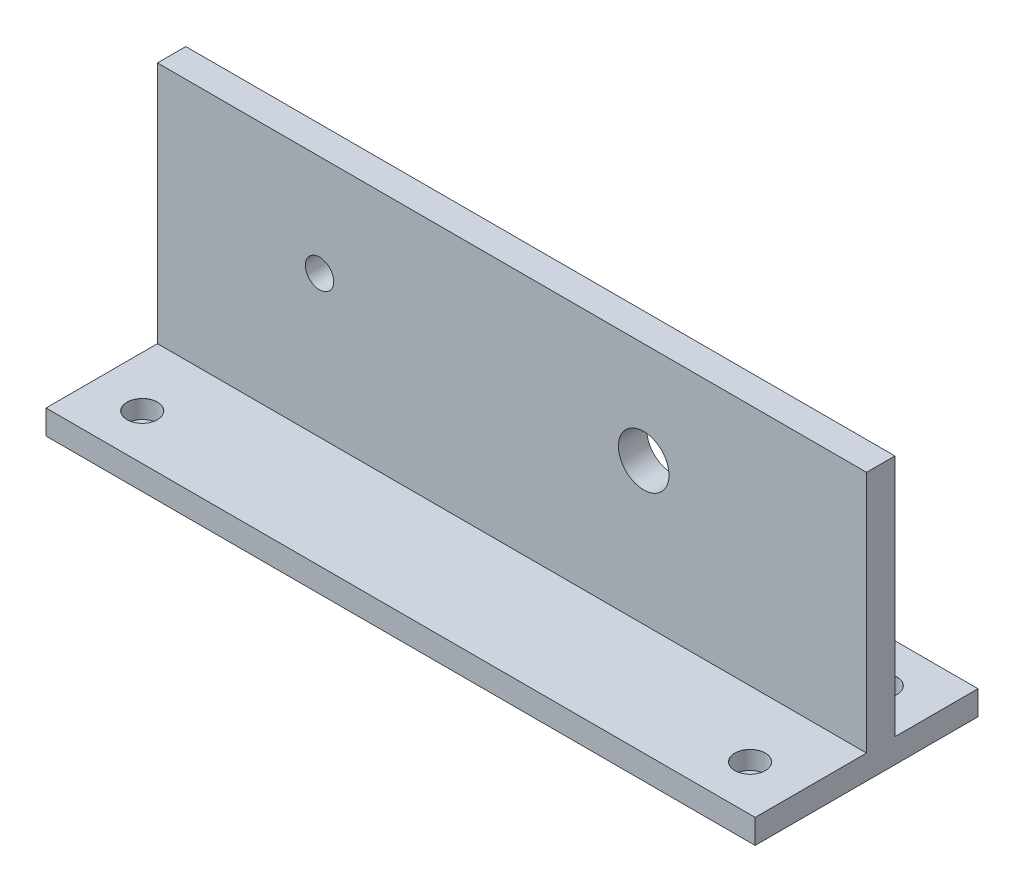
from build123d import *

# Parameters (mm, degrees)
SKETCH1_W                                    = 350
SKETCH1_H                                    = 110
BOSS_EXTRUDE1_DEPTH                          = 12
SKETCH2_W                                    = 350
SKETCH2_H                                    = 14
BOSS_EXTRUDE2_DEPTH                          = 120
CBORE_FOR_M8_HEXAGON_SOCKET_HEAD_CAP_2_COUNT = 2
CBORE_FOR_M8_HEXAGON_SOCKET_HEAD_CAP_2_PITCH = 65
CBORE_FOR_M8_HEXAGON_SOCKET_HEAD_CAP_3_COUNT = 2
CBORE_FOR_M8_HEXAGON_SOCKET_HEAD_CAP_3_PITCH = 300
CBORE_FOR_M8_HEXAGON_SOCKET_HEAD_CAP_4_COUNT = 2
CBORE_FOR_M8_HEXAGON_SOCKET_HEAD_CAP_4_PITCH = 306.960909563
CUT_EXTRUDE1_DEPTH                           = 230.804264538
CUT_EXTRUDE1_DEPTH_BACK                      = 230.804264538
SKETCH6_R                                    = 7
CUT_EXTRUDE2_DEPTH                           = 230.804264538
CUT_EXTRUDE2_DEPTH_BACK                      = 230.804264538
SKETCH7_R                                    = 12.5


with BuildPart() as part:
    # Sketch1 → Boss-Extrude1 (new body)
    with BuildSketch(Plane(origin=(0, 0, 0), x_dir=(1, 0, 0), z_dir=(0, 1, 0))):
        Rectangle(SKETCH1_W, SKETCH1_H)
    extrude(amount=BOSS_EXTRUDE1_DEPTH)

    # Sketch2 → Boss-Extrude2 (add)
    with BuildSketch(Plane(origin=(0, 12, 0), x_dir=(1, 0, 0), z_dir=(0, 1, 0))):
        with Locations((0, 7)):
            Rectangle(SKETCH2_W, SKETCH2_H)
    extrude(amount=BOSS_EXTRUDE2_DEPTH)

    # Sketch4 → CBORE for M8 Hexagon socket head cap screws1 (revolve, cut)
    with BuildSketch(Plane(origin=(-150, 12, -32.5), x_dir=(0, 0, 1), z_dir=(1, 0, 0))):
        Polygon((0, 0), (0, 15.103872786), (4.5, 12.4), (4.5, 9), (7.5, 9), (7.5, 0.025), (7.525, 0), align=None)
    cbore_for_m8_hexagon_socket_head_cap_scr = revolve(axis=Axis((-150, 18.35, -32.5), (0, -1, 0)), mode=Mode.SUBTRACT)

    # CBORE for M8 Hexagon socket head cap 2: CBORE for M8 Hexagon socket head cap screws1 ×2
    with Locations(*[(0, 0, i * CBORE_FOR_M8_HEXAGON_SOCKET_HEAD_CAP_2_PITCH) for i in range(1, CBORE_FOR_M8_HEXAGON_SOCKET_HEAD_CAP_2_COUNT)]):
        add(cbore_for_m8_hexagon_socket_head_cap_scr, mode=Mode.SUBTRACT)

    # CBORE for M8 Hexagon socket head cap 3: CBORE for M8 Hexagon socket head cap screws1 ×2
    with Locations(*[(i * CBORE_FOR_M8_HEXAGON_SOCKET_HEAD_CAP_3_PITCH, 0, 0) for i in range(1, CBORE_FOR_M8_HEXAGON_SOCKET_HEAD_CAP_3_COUNT)]):
        add(cbore_for_m8_hexagon_socket_head_cap_scr, mode=Mode.SUBTRACT)

    # CBORE for M8 Hexagon socket head cap 4: CBORE for M8 Hexagon socket head cap screws1 ×2
    with Locations(*[Vector(0.9773231400267972, 0, 0.21175334700580606) * (i * CBORE_FOR_M8_HEXAGON_SOCKET_HEAD_CAP_4_PITCH) for i in range(1, CBORE_FOR_M8_HEXAGON_SOCKET_HEAD_CAP_4_COUNT)]):
        add(cbore_for_m8_hexagon_socket_head_cap_scr, mode=Mode.SUBTRACT)

    # Sketch6 → Cut-Extrude1 (cut, two sides: drawn at the far end of the back side and taken through both)
    with BuildSketch(Plane(origin=(0, 0, -14), x_dir=(-1, 0, 0), z_dir=(0, 0, -1)).offset(-CUT_EXTRUDE1_DEPTH_BACK)):
        with Locations((95, 82)):
            Circle(SKETCH6_R)
    extrude(amount=CUT_EXTRUDE1_DEPTH + CUT_EXTRUDE1_DEPTH_BACK, mode=Mode.SUBTRACT)

    # Sketch7 → Cut-Extrude2 (cut, two sides: drawn at the far end of the back side and taken through both)
    with BuildSketch(Plane(origin=(0, 0, -14), x_dir=(-1, 0, 0), z_dir=(0, 0, -1)).offset(-CUT_EXTRUDE2_DEPTH_BACK)):
        with Locations((-65, 82)):
            Circle(SKETCH7_R)
    extrude(amount=CUT_EXTRUDE2_DEPTH + CUT_EXTRUDE2_DEPTH_BACK, mode=Mode.SUBTRACT)


solid = part.part
